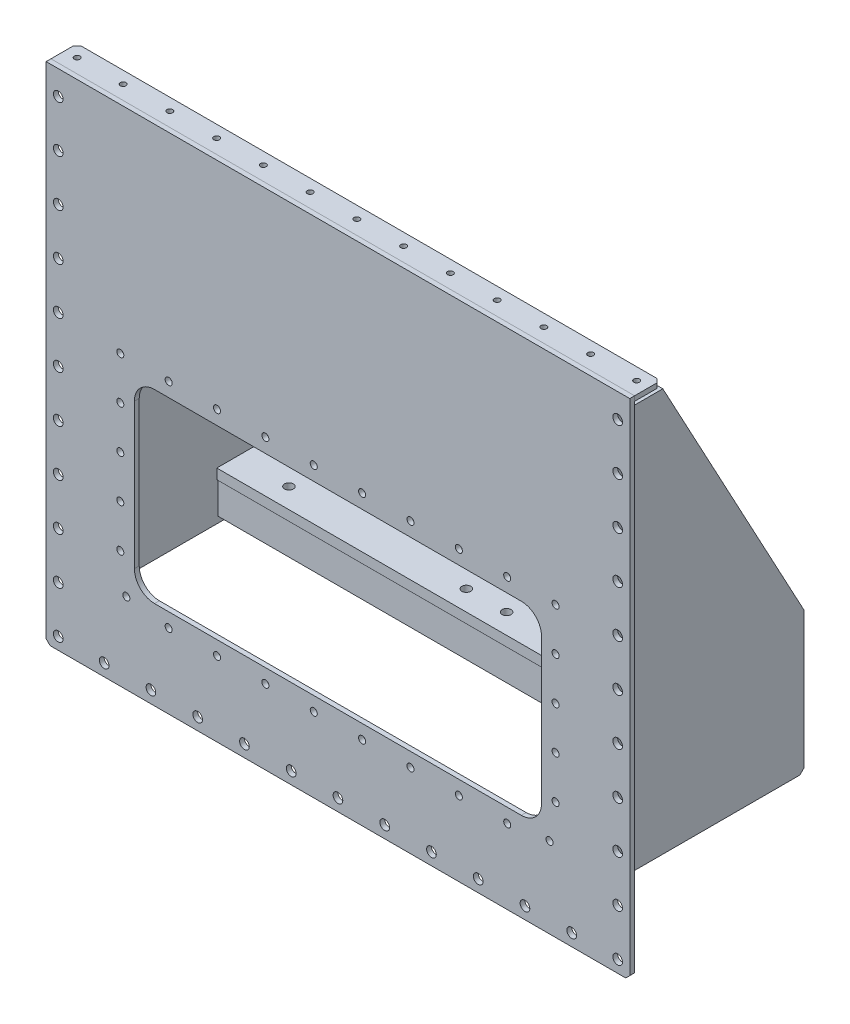
from build123d import *

# Parameters (mm, degrees)
SKETCH1_W                  = 1448
SKETCH1_H                  = 1250
BOSS_EXTRUDE1_DEPTH        = 12
SKETCH2_W                  = 1010
SKETCH2_H                  = 460
CUT_EXTRUDE1_DEPTH         = 12
FILLET1_R                  = 50
CHAMFER1_SIZE              = 10
SKETCH3_W                  = 1448
SKETCH3_H                  = 12
BOSS_EXTRUDE2_DEPTH        = 65
SKETCH4_R                  = 12
CUT_EXTRUDE2_DEPTH         = 12
LPATTERN1_COUNT            = 5
LPATTERN1_PITCH            = 106
SKETCH10_W                 = 12
SKETCH10_H                 = 480
BOSS_EXTRUDE3_DEPTH        = 50
CHAMFER2_SIZE              = 30
LPATTERN5_COUNT            = 2
LPATTERN5_PITCH            = 342
CHAMFER3_SIZE              = 10
SKETCH11_W                 = 12
SKETCH11_H                 = 142
BOSS_EXTRUDE4_DEPTH        = 50
CHAMFER4_SIZE              = 30
LPATTERN6_COUNT            = 2
LPATTERN6_PITCH            = 342
SKETCH12_R                 = 7
CUT_EXTRUDE3_DEPTH         = 12
SKETCH13_R                 = 7
CUT_EXTRUDE4_DEPTH         = 12
SKETCH14_R                 = 7
BOSS_EXTRUDE5_DEPTH        = 12
LPATTERN7_COUNT            = 2
LPATTERN7_PITCH            = 114
LPATTERN8_COUNT            = 11
LPATTERN8_PITCH            = 116
LPATTERN10_COUNT           = 2
LPATTERN10_PITCH           = 114
LPATTERN11_COUNT           = 9
LPATTERN11_PITCH           = 120
LPATTERN12_COUNT           = 8
LPATTERN12_PITCH           = 120
SKETCH22_W                 = 25
SKETCH22_H                 = 1000
BOSS_EXTRUDE6_DEPTH        = 500
CUT_EXTRUDE5_DEPTH         = 25
CHAMFER5_SIZE              = 10
CHAMFER5_OF_MIRROR6_SIZE   = 10
SKETCH27_W                 = 1240.908789267
SKETCH27_H                 = 180
BOSS_EXTRUDE7_DEPTH        = 25
SKETCH28_W                 = 1238
SKETCH28_H                 = 20
BOSS_EXTRUDE8_DEPTH        = 80
SKETCH29_W                 = 1238
SKETCH29_H                 = 20
BOSS_EXTRUDE9_DEPTH        = 80
SKETCH33_W                 = 11
SKETCH33_H                 = 25.001
F_22_0_22_HOLE2_AT_2_COUNT = 2
F_22_0_22_HOLE2_AT_2_PITCH = 80
F_22_0_22_HOLE2_AT_3_COUNT = 2
F_22_0_22_HOLE2_AT_3_PITCH = 440
F_22_0_22_HOLE2_AT_4_COUNT = 2
F_22_0_22_HOLE2_AT_4_PITCH = 447.2135955
F_22_0_22_HOLE2_AT_5_COUNT = 2
F_22_0_22_HOLE2_AT_5_PITCH = 983.259884263
F_22_0_22_HOLE2_AT_6_COUNT = 2
F_22_0_22_HOLE2_AT_6_PITCH = 545.893762558
F_22_0_22_HOLE2_AT_7_COUNT = 2
F_22_0_22_HOLE2_AT_7_PITCH = 980
F_22_0_22_HOLE2_AT_8_COUNT = 2
F_22_0_22_HOLE2_AT_8_PITCH = 540


with BuildPart() as part:
    # Sketch1 → Boss-Extrude1 (new body)
    with BuildSketch(Plane.XY):
        with Locations((645.959077371, 535.721184513)):
            Rectangle(SKETCH1_W, SKETCH1_H)
    extrude(amount=BOSS_EXTRUDE1_DEPTH)

    # Sketch2 → Cut-Extrude1 (cut)
    with BuildSketch(Plane(origin=(0, 0, 0), x_dir=(-1, 0, 0), z_dir=(0, 0, -1))):
        with Locations((-645.959077371, 360.721184513)):
            Rectangle(SKETCH2_W, SKETCH2_H)
    extrude(amount=-CUT_EXTRUDE1_DEPTH, mode=Mode.SUBTRACT)

    # Fillet1
    fillet1_edges = [part.edges().sort_by_distance(p)[0] for p in [
        (1150.959077371, 130.721184513, 6),
        (1150.959077371, 590.721184513, 6),
        (140.959077371, 590.721184513, 6),
        (140.959077371, 130.721184513, 6),
    ]]
    fillet(fillet1_edges, radius=FILLET1_R)

    # Chamfer1
    chamfer1_edges = [part.edges().sort_by_distance(p)[0] for p in [
        (1369.959077371, -89.278815487, 6),
        (-78.040922629, -89.278815487, 6),
    ]]
    chamfer(chamfer1_edges, length=CHAMFER1_SIZE)

    # Sketch4 → Cut-Extrude2 (cut)
    with BuildSketch(Plane(origin=(0, 0, 0), x_dir=(-1, 0, 0), z_dir=(0, 0, -1))):
        with Locations((-1339.959077371, 1100.721184513)):
            Circle(SKETCH4_R)
        with Locations((-1339.959077371, 984.721184513)):
            Circle(SKETCH4_R)
        with Locations((-1339.959077371, 868.721184513)):
            Circle(SKETCH4_R)
        with Locations((-1339.959077371, 752.721184513)):
            Circle(SKETCH4_R)
        with Locations((-1339.959077371, 636.721184513)):
            Circle(SKETCH4_R)
        with Locations((-1339.959077371, 520.721184513)):
            Circle(SKETCH4_R)
        with Locations((-1339.959077371, 404.721184513)):
            Circle(SKETCH4_R)
        with Locations((-1339.959077371, 288.721184513)):
            Circle(SKETCH4_R)
        with Locations((-1339.959077371, 172.721184513)):
            Circle(SKETCH4_R)
        with Locations((-1339.959077371, 56.721184513)):
            Circle(SKETCH4_R)
        with Locations((-1339.959077371, -59.278815487)):
            Circle(SKETCH4_R)
        with Locations(Location((48.040922629, -59.278815487, 0), (0, 0, 180))):
            Circle(SKETCH4_R)
        with Locations(Location((48.040922629, 56.721184513, 0), (0, 0, 180))):
            Circle(SKETCH4_R)
        with Locations(Location((48.040922629, 172.721184513, 0), (0, 0, 180))):
            Circle(SKETCH4_R)
        with Locations(Location((48.040922629, 288.721184513, 0), (0, 0, 180))):
            Circle(SKETCH4_R)
        with Locations(Location((48.040922629, 404.721184513, 0), (0, 0, 180))):
            Circle(SKETCH4_R)
        with Locations(Location((48.040922629, 520.721184513, 0), (0, 0, 180))):
            Circle(SKETCH4_R)
        with Locations(Location((48.040922629, 636.721184513, 0), (0, 0, 180))):
            Circle(SKETCH4_R)
        with Locations(Location((48.040922629, 752.721184513, 0), (0, 0, 180))):
            Circle(SKETCH4_R)
        with Locations(Location((48.040922629, 868.721184513, 0), (0, 0, 180))):
            Circle(SKETCH4_R)
        with Locations(Location((48.040922629, 984.721184513, 0), (0, 0, 180))):
            Circle(SKETCH4_R)
        with Locations(Location((48.040922629, 1100.721184513, 0), (0, 0, 180))):
            Circle(SKETCH4_R)
        with Locations((-1225.959077371, -59.278815487)):
            Circle(SKETCH4_R)
        with Locations((-1109.959077371, -59.278815487)):
            Circle(SKETCH4_R)
        with Locations((-993.959077371, -59.278815487)):
            Circle(SKETCH4_R)
        with Locations((-877.959077371, -59.278815487)):
            Circle(SKETCH4_R)
        with Locations((-761.959077371, -59.278815487)):
            Circle(SKETCH4_R)
        with Locations((-645.959077371, -59.278815487)):
            Circle(SKETCH4_R)
        with Locations((-529.959077371, -59.278815487)):
            Circle(SKETCH4_R)
        with Locations((-413.959077371, -59.278815487)):
            Circle(SKETCH4_R)
        with Locations((-297.959077371, -59.278815487)):
            Circle(SKETCH4_R)
        with Locations((-181.959077371, -59.278815487)):
            Circle(SKETCH4_R)
        with Locations((-65.959077371, -59.278815487)):
            Circle(SKETCH4_R)
    extrude(amount=-CUT_EXTRUDE2_DEPTH, mode=Mode.SUBTRACT)

    # Sketch6 → M20 Tapped Hole1 (revolve, cut)
    with BuildSketch(Plane(origin=(1185.959077371, 625.721184513, 0), x_dir=(0, 1, 0), z_dir=(1, 0, 0))):
        Polygon((0, 0), (0, 57.757530416), (8.75, 52.5), (8.75, 0), align=None)
    m20_tapped_hole1 = revolve(axis=Axis((1185.959077371, 625.721184513, -6.35), (0, 0, 1)), mode=Mode.SUBTRACT)

    # LPattern1: M20 Tapped Hole1 ×5
    with Locations(*[(0, -i * LPATTERN1_PITCH, 0) for i in range(1, LPATTERN1_COUNT)]):
        add(m20_tapped_hole1, mode=Mode.SUBTRACT)

    # Mirror1: M20 Tapped Hole1 across plane
    add(m20_tapped_hole1.mirror(Plane.ZY.offset(-645.959077371)), mode=Mode.SUBTRACT)

    # Mirror1 copy 1 sketch → Mirror1 copy 1 (revolve, cut)
    with BuildSketch(Plane(origin=(105.959077371, 519.721184513, 0), x_dir=(0, 1, 0), z_dir=(-1, 0, 0))):
        Polygon((0, 0), (0, -57.757530416), (8.75, -52.5), (8.75, 0), align=None)
    revolve(axis=Axis((105.959077371, 519.721184513, -6.35), (0, 0, -1)), mode=Mode.SUBTRACT)

    # Mirror1 copy 2 sketch → Mirror1 copy 2 (revolve, cut)
    with BuildSketch(Plane(origin=(105.959077371, 413.721184513, 0), x_dir=(0, 1, 0), z_dir=(-1, 0, 0))):
        Polygon((0, 0), (0, -57.757530416), (8.75, -52.5), (8.75, 0), align=None)
    revolve(axis=Axis((105.959077371, 413.721184513, -6.35), (0, 0, -1)), mode=Mode.SUBTRACT)

    # Mirror1 copy 3 sketch → Mirror1 copy 3 (revolve, cut)
    with BuildSketch(Plane(origin=(105.959077371, 307.721184513, 0), x_dir=(0, 1, 0), z_dir=(-1, 0, 0))):
        Polygon((0, 0), (0, -57.757530416), (8.75, -52.5), (8.75, 0), align=None)
    revolve(axis=Axis((105.959077371, 307.721184513, -6.35), (0, 0, -1)), mode=Mode.SUBTRACT)

    # Mirror1 copy 4 sketch → Mirror1 copy 4 (revolve, cut)
    with BuildSketch(Plane(origin=(105.959077371, 201.721184513, 0), x_dir=(0, 1, 0), z_dir=(-1, 0, 0))):
        Polygon((0, 0), (0, -57.757530416), (8.75, -52.5), (8.75, 0), align=None)
    revolve(axis=Axis((105.959077371, 201.721184513, -6.35), (0, 0, -1)), mode=Mode.SUBTRACT)

    # LPattern11: M20 Tapped Hole1 ×9
    with Locations(*[(-i * LPATTERN11_PITCH, 0, 0) for i in range(1, LPATTERN11_COUNT)]):
        add(m20_tapped_hole1, mode=Mode.SUBTRACT)

    # Sketch16 → M20 Tapped Hole2 (revolve, cut)
    with BuildSketch(Plane(origin=(1170.959077371, 110.721184513, 0), x_dir=(0, 1, 0), z_dir=(1, 0, 0))):
        Polygon((0, 0), (0, 57.757530416), (8.75, 52.5), (8.75, 0), align=None)
    m20_tapped_hole2 = revolve(axis=Axis((1170.959077371, 110.721184513, -6.35), (0, 0, 1)), mode=Mode.SUBTRACT)

    # Mirror5: M20 Tapped Hole2 across plane
    add(m20_tapped_hole2.mirror(Plane.ZY.offset(-645.959077371)), mode=Mode.SUBTRACT)

    # Sketch19 → M20 Tapped Hole3 (revolve, cut)
    with BuildSketch(Plane(origin=(1065.959077371, 95.721184513, 0), x_dir=(0, 1, 0), z_dir=(1, 0, 0))):
        Polygon((0, 0), (0, 57.757530416), (8.75, 52.5), (8.75, 0), align=None)
    m20_tapped_hole3 = revolve(axis=Axis((1065.959077371, 95.721184513, -6.35), (0, 0, 1)), mode=Mode.SUBTRACT)

    # LPattern12: M20 Tapped Hole3 ×8
    with Locations(*[(-i * LPATTERN12_PITCH, 0, 0) for i in range(1, LPATTERN12_COUNT)]):
        add(m20_tapped_hole3, mode=Mode.SUBTRACT)

    # Sketch22 → Boss-Extrude6 (add)
    with BuildSketch(Plane(origin=(0, 0, 0), x_dir=(-1, 0, 0), z_dir=(0, 0, -1))):
        with Locations((-1277.459077371, 560.721184513)):
            Rectangle(SKETCH22_W, SKETCH22_H)
    boss_extrude6 = extrude(amount=BOSS_EXTRUDE6_DEPTH)

    # Sketch23 → Cut-Extrude5 (cut)
    with BuildSketch(Plane(origin=(1289.959077371, 0, 0), x_dir=(0, 0, -1), z_dir=(1, 0, 0))):
        Polygon((150, 1060.721184513), (500, 410.721184513), (500, 1060.721184513), align=None)
    cut_extrude5 = extrude(amount=-CUT_EXTRUDE5_DEPTH, mode=Mode.SUBTRACT)

    # Chamfer5
    chamfer5_edges = [part.edges().sort_by_distance(p)[0] for p in [
        (1277.459077371, 60.721184513, -500),
    ]]
    chamfer(chamfer5_edges, length=CHAMFER5_SIZE)

    # Mirror6: Boss-Extrude6, Cut-Extrude5 across plane
    add(boss_extrude6.mirror(Plane.ZY.offset(-645.959077371)))
    add(cut_extrude5.mirror(Plane.ZY.offset(-645.959077371)), mode=Mode.SUBTRACT)

    # Chamfer5 of Mirror6
    chamfer5_of_mirror6_edges = [part.edges().sort_by_distance(p)[0] for p in [
        (14.459077371, 60.721184513, -500),
    ]]
    chamfer(chamfer5_of_mirror6_edges, length=CHAMFER5_OF_MIRROR6_SIZE)


with BuildPart() as body_2:
    # Sketch3 → Boss-Extrude2 (new body)
    with BuildSketch(Plane(origin=(0, 0, 0), x_dir=(-1, 0, 0), z_dir=(0, 0, -1))):
        with Locations((-645.959077371, 1154.721184513)):
            Rectangle(SKETCH3_W, SKETCH3_H)
    extrude(amount=BOSS_EXTRUDE2_DEPTH)

    # Chamfer3
    chamfer3_edges = [body_2.edges().sort_by_distance(p)[0] for p in [
        (-78.040922629, 1154.721184513, -65),
        (1369.959077371, 1154.721184513, -65),
    ]]
    chamfer(chamfer3_edges, length=CHAMFER3_SIZE)

    # Sketch12 → Cut-Extrude3 (cut)
    with BuildSketch(Plane(origin=(0, 1160.721184513, 0), x_dir=(1, 0, 0), z_dir=(0, 1, 0))):
        with Locations(Location((1339.959077371, 35, 0), (0, 0, 270))):
            Circle(SKETCH12_R)
    extrude(amount=-CUT_EXTRUDE3_DEPTH, mode=Mode.SUBTRACT)

    # Sketch13 → Cut-Extrude4 (cut)
    with BuildSketch(Plane(origin=(0, 1160.721184513, 0), x_dir=(1, 0, 0), z_dir=(0, 1, 0))):
        with Locations(Location((-48.040922629, 35, 0), (0, 0, 270))):
            Circle(SKETCH13_R)
        with Locations(Location((65.959077371, 35, 0), (0, 0, 270))):
            Circle(SKETCH13_R)
        with Locations(Location((181.959077371, 35, 0), (0, 0, 270))):
            Circle(SKETCH13_R)
        with Locations(Location((297.959077371, 35, 0), (0, 0, 270))):
            Circle(SKETCH13_R)
        with Locations(Location((413.959077371, 35, 0), (0, 0, 270))):
            Circle(SKETCH13_R)
        with Locations(Location((529.959077371, 35, 0), (0, 0, 270))):
            Circle(SKETCH13_R)
        with Locations(Location((645.959077371, 35, 0), (0, 0, 270))):
            Circle(SKETCH13_R)
        with Locations(Location((761.959077371, 35, 0), (0, 0, 270))):
            Circle(SKETCH13_R)
        with Locations(Location((877.959077371, 35, 0), (0, 0, 270))):
            Circle(SKETCH13_R)
        with Locations(Location((993.959077371, 35, 0), (0, 0, 270))):
            Circle(SKETCH13_R)
        with Locations(Location((1109.959077371, 35, 0), (0, 0, 270))):
            Circle(SKETCH13_R)
        with Locations(Location((1225.959077371, 35, 0), (0, 0, 270))):
            Circle(SKETCH13_R)
    extrude(amount=-CUT_EXTRUDE4_DEPTH, mode=Mode.SUBTRACT)


with BuildPart() as body_3:
    # Sketch10 → Boss-Extrude3 (new body)
    with BuildSketch(Plane(origin=(0, 0, 0), x_dir=(-1, 0, 0), z_dir=(0, 0, -1))):
        with Locations((-822.959077371, 908.721184513)):
            Rectangle(SKETCH10_W, SKETCH10_H)
    extrude(amount=BOSS_EXTRUDE3_DEPTH)

    # Chamfer2
    chamfer2_edges = [body_3.edges().sort_by_distance(p)[0] for p in [
        (822.959077371, 668.721184513, -50),
    ]]
    chamfer(chamfer2_edges, length=CHAMFER2_SIZE)


with BuildPart() as lpattern5_1:
    # LPattern5: pattern copy
    add(body_3.part.moved(Location(Vector(1, 0, 0) * (1 * LPATTERN5_PITCH))))


with BuildPart() as body_5:
    # Mirror3: mirrored copy
    add(lpattern5_1.part.mirror(Plane.ZY.offset(-645.959077371)))


with BuildPart() as body_6:
    # Mirror3 2: mirrored copy
    add(body_3.part.mirror(Plane.ZY.offset(-645.959077371)))


with BuildPart() as body_7:
    # Sketch11 → Boss-Extrude4 (new body)
    with BuildSketch(Plane(origin=(0, 0, 0), x_dir=(-1, 0, 0), z_dir=(0, 0, -1))):
        with Locations((-822.959077371, -18.278815487)):
            Rectangle(SKETCH11_W, SKETCH11_H)
    extrude(amount=BOSS_EXTRUDE4_DEPTH)

    # Chamfer4
    chamfer4_edges = [body_7.edges().sort_by_distance(p)[0] for p in [
        (822.959077371, 52.721184513, -50),
    ]]
    chamfer(chamfer4_edges, length=CHAMFER4_SIZE)


with BuildPart() as lpattern6_1:
    # LPattern6: pattern copy
    add(body_7.part.moved(Location(Vector(1, 0, 0) * (1 * LPATTERN6_PITCH))))


with BuildPart() as body_9:
    # Mirror4: mirrored copy
    add(lpattern6_1.part.mirror(Plane.ZY.offset(-645.959077371)))


with BuildPart() as body_10:
    # Mirror4 2: mirrored copy
    add(body_7.part.mirror(Plane.ZY.offset(-645.959077371)))


with BuildPart() as body_11:
    # Sketch14 → Boss-Extrude5 (new body)
    with BuildSketch(Plane.XZ.offset(-1148.721184513)):
        Polygon((-34.287762693, -35), (-41.164342661, -23.089414113), (-54.917502597, -23.089414113), (-61.794082565, -35), (-54.917502597, -46.910585887), (-41.164342661, -46.910585887), align=None)
        with Locations(Location((-48.040922629, -35, 0), (0, 0, 270))):
            Circle(SKETCH14_R, mode=Mode.SUBTRACT)
    boss_extrude5 = extrude(amount=BOSS_EXTRUDE5_DEPTH)


with BuildPart() as lpattern7_1:
    # LPattern7: Boss-Extrude5 ×2
    with Locations(*[(i * LPATTERN7_PITCH, 0, 0) for i in range(1, LPATTERN7_COUNT)]):
        add(boss_extrude5)


with BuildPart() as lpattern8_1:
    # LPattern8: pattern copy
    add(lpattern7_1.part.moved(Location(Vector(1, 0, 0) * (1 * LPATTERN8_PITCH))))


with BuildPart() as lpattern8_2:
    # LPattern8: pattern copy
    add(lpattern7_1.part.moved(Location(Vector(1, 0, 0) * (2 * LPATTERN8_PITCH))))


with BuildPart() as lpattern8_3:
    # LPattern8: pattern copy
    add(lpattern7_1.part.moved(Location(Vector(1, 0, 0) * (3 * LPATTERN8_PITCH))))


with BuildPart() as lpattern8_4:
    # LPattern8: pattern copy
    add(lpattern7_1.part.moved(Location(Vector(1, 0, 0) * (4 * LPATTERN8_PITCH))))


with BuildPart() as lpattern8_5:
    # LPattern8: pattern copy
    add(lpattern7_1.part.moved(Location(Vector(1, 0, 0) * (5 * LPATTERN8_PITCH))))


with BuildPart() as lpattern8_6:
    # LPattern8: pattern copy
    add(lpattern7_1.part.moved(Location(Vector(1, 0, 0) * (6 * LPATTERN8_PITCH))))


with BuildPart() as lpattern8_7:
    # LPattern8: pattern copy
    add(lpattern7_1.part.moved(Location(Vector(1, 0, 0) * (7 * LPATTERN8_PITCH))))


with BuildPart() as lpattern8_8:
    # LPattern8: pattern copy
    add(lpattern7_1.part.moved(Location(Vector(1, 0, 0) * (8 * LPATTERN8_PITCH))))


with BuildPart() as lpattern8_9:
    # LPattern8: pattern copy
    add(lpattern7_1.part.moved(Location(Vector(1, 0, 0) * (9 * LPATTERN8_PITCH))))


with BuildPart() as lpattern8_10:
    # LPattern8: pattern copy
    add(lpattern7_1.part.moved(Location(Vector(1, 0, 0) * (10 * LPATTERN8_PITCH))))


with BuildPart() as lpattern10_1:
    # LPattern10: pattern copy
    add(lpattern8_10.part.moved(Location(Vector(1, 0, 0) * (1 * LPATTERN10_PITCH))))


with BuildPart() as body_24:
    # Sketch27 → Boss-Extrude7 (new body)
    with BuildSketch(Plane(origin=(-4.624027257, 180.721184513, 0), x_dir=(1, 0, 0), z_dir=(0, -1, 0))):
        with Locations((649.128709995, -396.500000002)):
            Rectangle(SKETCH27_W, SKETCH27_H)
    extrude(amount=BOSS_EXTRUDE7_DEPTH)

    # Sketch33 → Ø22.0 (22) Hole2 (revolve, cut)
    with BuildSketch(Plane(origin=(1135.959077371, 180.721184513, -356.5), x_dir=(0, 0, 1), z_dir=(1, 0, 0))):
        with Locations((5.5, 12.5005)):
            Rectangle(SKETCH33_W, SKETCH33_H)
    f_22_0_22_hole2 = revolve(axis=Axis((1135.959077371, 187.071184513, -356.5), (0, -1, 0)), mode=Mode.SUBTRACT)

    # Ø22.0 (22) Hole2 at 2: Ø22.0 (22) Hole2 ×2
    with Locations(*[(0, 0, -i * F_22_0_22_HOLE2_AT_2_PITCH) for i in range(1, F_22_0_22_HOLE2_AT_2_COUNT)]):
        add(f_22_0_22_hole2, mode=Mode.SUBTRACT)

    # Ø22.0 (22) Hole2 at 3: Ø22.0 (22) Hole2 ×2
    with Locations(*[(-i * F_22_0_22_HOLE2_AT_3_PITCH, 0, 0) for i in range(1, F_22_0_22_HOLE2_AT_3_COUNT)]):
        add(f_22_0_22_hole2, mode=Mode.SUBTRACT)

    # Ø22.0 (22) Hole2 at 4: Ø22.0 (22) Hole2 ×2
    with Locations(*[Vector(-0.9838699100999064, 0, -0.17888543819998917) * (i * F_22_0_22_HOLE2_AT_4_PITCH) for i in range(1, F_22_0_22_HOLE2_AT_4_COUNT)]):
        add(f_22_0_22_hole2, mode=Mode.SUBTRACT)

    # Ø22.0 (22) Hole2 at 5: Ø22.0 (22) Hole2 ×2
    with Locations(*[Vector(-0.9966846158226085, 0, -0.08136200945490113) * (i * F_22_0_22_HOLE2_AT_5_PITCH) for i in range(1, F_22_0_22_HOLE2_AT_5_COUNT)]):
        add(f_22_0_22_hole2, mode=Mode.SUBTRACT)

    # Ø22.0 (22) Hole2 at 6: Ø22.0 (22) Hole2 ×2
    with Locations(*[Vector(-0.9892034623538727, 0, -0.1465486610894501) * (i * F_22_0_22_HOLE2_AT_6_PITCH) for i in range(1, F_22_0_22_HOLE2_AT_6_COUNT)]):
        add(f_22_0_22_hole2, mode=Mode.SUBTRACT)

    # Ø22.0 (22) Hole2 at 7: Ø22.0 (22) Hole2 ×2
    with Locations(*[(-i * F_22_0_22_HOLE2_AT_7_PITCH, 0, 0) for i in range(1, F_22_0_22_HOLE2_AT_7_COUNT)]):
        add(f_22_0_22_hole2, mode=Mode.SUBTRACT)

    # Ø22.0 (22) Hole2 at 8: Ø22.0 (22) Hole2 ×2
    with Locations(*[(-i * F_22_0_22_HOLE2_AT_8_PITCH, 0, 0) for i in range(1, F_22_0_22_HOLE2_AT_8_COUNT)]):
        add(f_22_0_22_hole2, mode=Mode.SUBTRACT)


with BuildPart() as body_25:
    # Sketch28 → Boss-Extrude8 (new body)
    with BuildSketch(Plane.XZ.offset(-155.721184513)):
        with Locations((645.959077371, -319.5)):
            Rectangle(SKETCH28_W, SKETCH28_H)
    extrude(amount=BOSS_EXTRUDE8_DEPTH)


with BuildPart() as body_26:
    # Sketch29 → Boss-Extrude9 (new body)
    with BuildSketch(Plane.XZ.offset(-155.721184513)):
        with Locations((645.959077371, -485)):
            Rectangle(SKETCH29_W, SKETCH29_H)
    extrude(amount=BOSS_EXTRUDE9_DEPTH)


solid = Compound([part.part, body_2.part, body_3.part, lpattern5_1.part, body_5.part, body_6.part, body_7.part, lpattern6_1.part, body_9.part, body_10.part, body_11.part, lpattern7_1.part, lpattern8_1.part, lpattern8_2.part, lpattern8_3.part, lpattern8_4.part, lpattern8_5.part, lpattern8_6.part, lpattern8_7.part, lpattern8_8.part, lpattern8_9.part, lpattern8_10.part, lpattern10_1.part, body_24.part, body_25.part, body_26.part])
